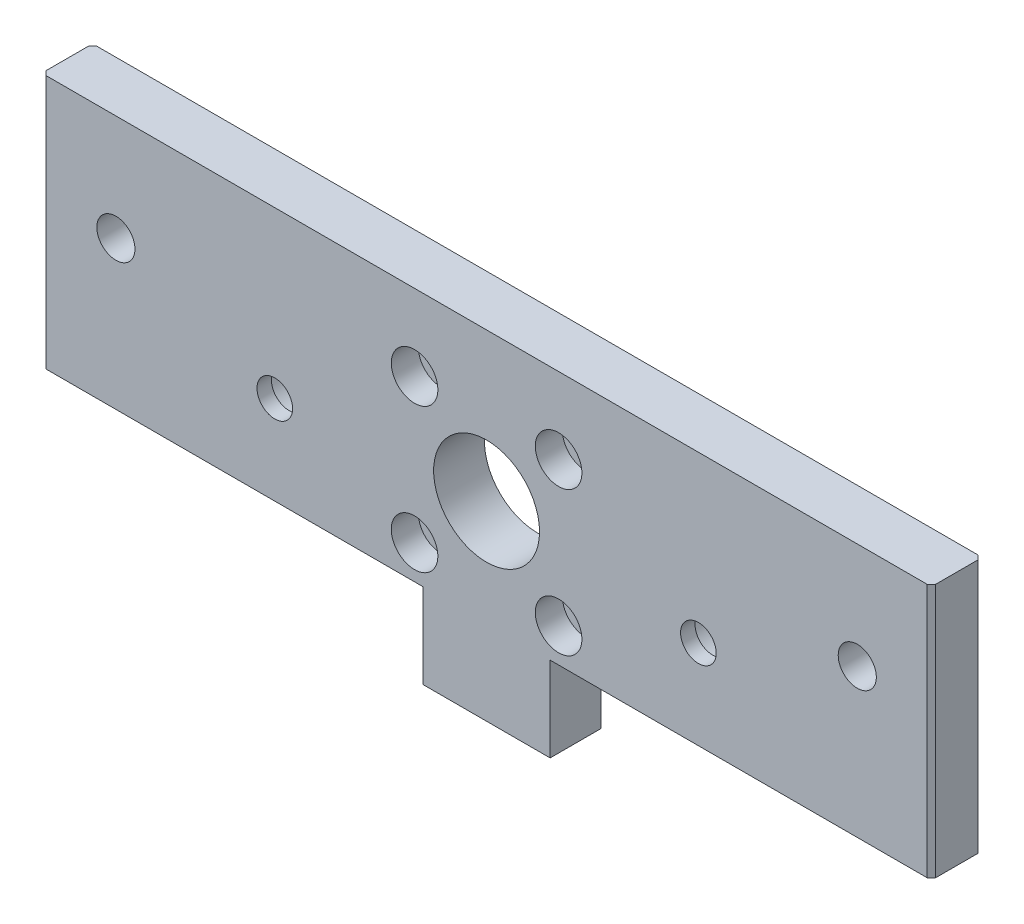
SolidWorks part; units mm, degrees
ref_plane "前视基准面" through (0, 0, 0) normal (0, 0, 1) x (1, 0, 0)
ref_plane "上视基准面" through (0, 0, 0) normal (0, 1, 0) x (1, 0, 0)
ref_plane "右视基准面" through (0, 0, 0) normal (1, 0, 0) x (0, 0, -1)
sketch "草图1" plane through (0, 0, 0) normal (0, 0, 1) x (1, 0, 0)
  line L1 (0, 0) -> (210, 0)
  line L2 (0, 0) -> (0, 60)
  line L3 (0, 60) -> (210, 60)
  line L4 (210, 0) -> (210, 60)
  dimension "D1" = 60
  dimension "D2" = 210
extrude "凸台-拉伸1" add sketch "草图1" along normal blind 12
sketch "草图2" plane through (0, 0, 12) normal (0, 0, 1) x (1, 0, 0)
  line L0 (105, 0) -> (105, 64.5324) construction
  line L1 (0, 0) -> (210, 0) construction
  circle A0 centre (105, 25) radius 12.5
  dimension "D1" = 25
  dimension "D2" = 25
extrude "切除-拉伸1" cut sketch "草图2" against normal blind 12
hole_wizard "M8 六角凹头螺钉的柱形沉头孔1" positions "草图6" profile "草图5" counterbore size "M8" standard "ISO" end condition through all
sketch "草图6" plane through (0, 0, 0) normal (0, 0, -1) x (-1, 0, 0)
  line L0 (-105, 0) -> (-105, 61.4062) construction
  line L1 (0, 0) -> (-210, 0) construction
  point P0 (-55, 21)
  point P3 (-155, 21)
  dimension "D1" = 21
  dimension "D2" = 100
sketch "草图5" plane through (55, 21, 0) normal (1, 0, 0) x (0, 1, 0)
  line L0 (0, 0) -> (0, 12)
  line L1 (0, 12) -> (4.2, 12)
  line L3 (4.2, 12) -> (4.2, 8.6)
  line L4 (4.2, 8.6) -> (7.5, 8.6)
  line L5 (7.5, 8.6) -> (7.5, 0)
  line L7 (7.5, 0) -> (0, 0)
  line L11 (0, -6.35) -> (0, 107.95) construction
  dimension "通孔孔直径" = 8.4
  dimension "通孔孔深度" = 12
  dimension "柱形沉头孔直径" = 15
  dimension "柱形沉头孔深度" = 8.6
ref_plane "基准面1" through (105, 0, 0) normal (1, 0, 0) x (0, 0, -1)
hole_wizard "M6 六角凹头螺钉的柱形沉头孔2" positions "草图10" profile "草图9" counterbore size "M6" standard "ISO" end condition through all
sketch "草图10" plane through (0, 0, 12) normal (0, 0, 1) x (1, 0, 0)
  line L0 (105, 0) -> (105, 54.8131) construction
  line L1 (105, -6.6) -> (105, 6.6) construction
  circle A0 centre (105, 25) radius 24.0416 construction
  point P0 (122, 42)
  point P3 (88, 42)
  point P6 (122, 8)
  point P9 (88, 8)
  dimension "D1" = 34
  dimension "D2" = 34
sketch "草图9" plane through (122, 42, 12) normal (1, 0, 0) x (0, -1, 0)
  line L0 (0, 0) -> (0, 12)
  line L1 (0, 12) -> (3.2, 12)
  line L3 (3.2, 12) -> (3.2, 6.4)
  line L4 (3.2, 6.4) -> (5.5, 6.4)
  line L5 (5.5, 6.4) -> (5.5, 0)
  line L7 (5.5, 0) -> (0, 0)
  line L11 (0, -6.35) -> (0, 107.95) construction
  dimension "通孔孔直径" = 6.4
  dimension "通孔孔深度" = 12
  dimension "柱形沉头孔直径" = 11
  dimension "柱形沉头孔深度" = 6.4
chamfer "倒角1" distance 1 angle 45 4 edges at (210, 30, 0) (210, 30, 12) (0, 30, 0) (0, 30, 12)
hole_wizard "Ø9.0 (9) 直径孔1" positions "草图11" profile "草图12" hole size "Ø9.0" standard "ISO" end condition through all
sketch "草图11" plane through (0, 0, 0) normal (0, 0, -1) x (-1, 0, 0)
  line L0 (-199, 35) -> (9.4509, 35) construction
  line L3 (-105, 60) -> (-105, -29.7955) construction
  line L4 (-209, 60) -> (-1, 60) construction
  line L5 (-105, 6.6) -> (-105, -6.6) construction
  point P0 (-192.5, 35)
  point P2 (-17.5, 35)
  dimension "D1" = 175
  dimension "D2" = 25
sketch "草图12" plane through (192.5, 35, 0) normal (1, 0, 0) x (0, 1, 0)
  line L0 (0, 0) -> (0, 12)
  line L1 (0, 12) -> (4.5, 12)
  line L2 (4.5, 12) -> (4.5, 0)
  line L5 (4.5, 0) -> (0, 0)
  line L11 (0, -6.35) -> (0, 107.95) construction
  dimension "通孔孔直径" = 9
  dimension "通孔孔深度" = 12
sketch "草图14" plane through (0, 0, 0) normal (0, 0, -1) x (-1, 0, 0)
  line L0 (-1, 0) -> (-209, 0) construction
  line L1 (-120, 0) -> (-90, 0)
  line L2 (-120, 0) -> (-120, -20)
  line L3 (-120, -20) -> (-90, -20)
  line L4 (-90, 0) -> (-90, -20)
  line L5 (-105, 27.1065) -> (-105, -63.2603) construction
  line L6 (-105, 6.6) -> (-105, -6.6) construction
  dimension "D1" = 30
  dimension "D2" = 20
extrude "凸台-拉伸2" add sketch "草图14" against normal up to surface (12 mm away) up to face at (188, 35, 12)
